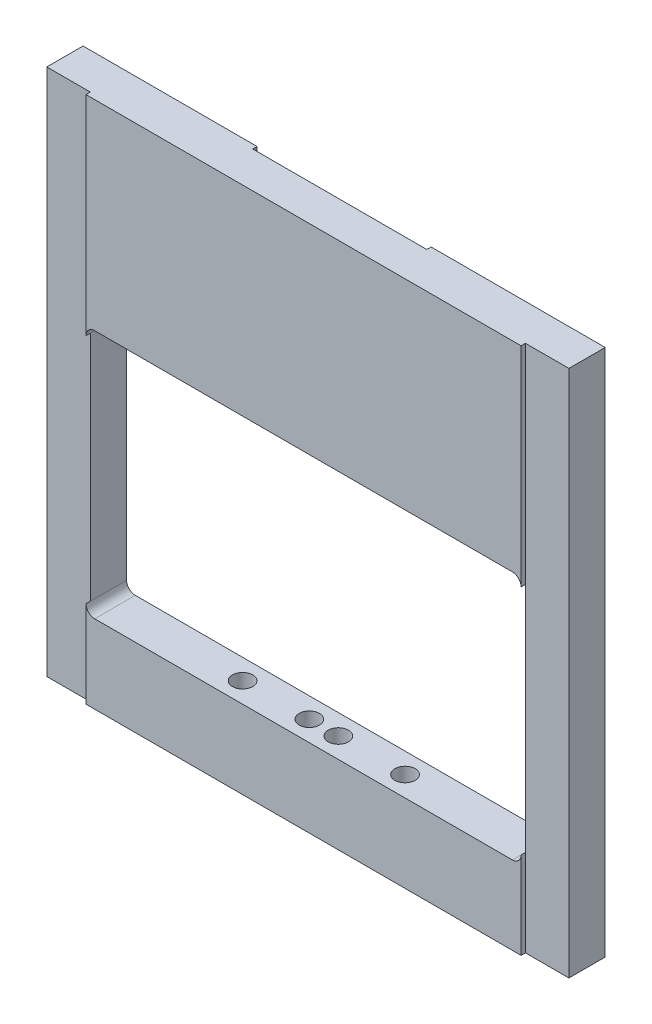
SolidWorks part; units mm, degrees
ref_plane "前视基准面" through (0, 0, 0) normal (0, 0, 1) x (1, 0, 0)
ref_plane "上视基准面" through (0, 0, 0) normal (0, 1, 0) x (1, 0, 0)
ref_plane "右视基准面" through (0, 0, 0) normal (1, 0, 0) x (0, 0, -1)
sketch "草图1" plane through (0, 0, 0) normal (0, 0, 1) x (1, 0, 0)
  line L1 (-90, -91) -> (90, -91)
  line L2 (-90, -91) -> (-90, 91)
  line L3 (-90, 91) -> (90, 91)
  line L4 (90, -91) -> (90, 91)
  line L5 (-90, -91) -> (90, 91) construction
  line L6 (-90, 91) -> (90, -91) construction
  point P0 (0, 0)
  dimension "D1" = 180
  dimension "D2" = 182
extrude "凸台-拉伸1" add sketch "草图1" along normal mid plane 14
sketch "草图2" plane through (0, 0, -7) normal (0, 0, -1) x (-1, 0, 0)
  line L0 (-90, 91) -> (90, 91) construction
  line L1 (-30, 27) -> (30, 27)
  line L2 (-30, 27) -> (-30, 91)
  line L3 (-30, 91) -> (30, 91)
  line L4 (30, 27) -> (30, 91)
  line L5 (-30, 27) -> (30, 91) construction
  line L6 (-30, 91) -> (30, 27) construction
  line L7 (90, -91) -> (-90, -91) construction
  line L8 (-30, -91) -> (30, -91)
  line L9 (-30, -91) -> (-30, -69)
  line L10 (-30, -69) -> (30, -69)
  line L11 (30, -91) -> (30, -69)
  line L12 (-30, -91) -> (30, -69) construction
  line L13 (-30, -69) -> (30, -91) construction
  point P0 (0, 59)
  point P7 (0, -80)
  dimension "D1" = 64
  dimension "D2" = 60
  dimension "D3" = 22
extrude "切除-拉伸1" cut sketch "草图2" against normal blind 1.5
sketch "草图3" plane through (0, 0, -7) normal (0, 0, -1) x (-1, 0, 0)
  line L0 (30, 27) -> (32, 27)
  line L1 (32, 37) -> (30, 37)
  line L2 (30, 27) -> (30, 91) construction
  line L3 (30, 37) -> (30, 27)
  line L9 (0, 0) -> (0, 27) construction
  line L10 (-30, 27) -> (30, 27) construction
  line L14 (-30, 37) -> (-30, 27)
  line L15 (-32, 37) -> (-30, 37)
  line L16 (-30, 27) -> (-32, 27)
  line L20 (30, -69) -> (32, -69)
  line L21 (32, -79) -> (30, -79)
  line L22 (30, -91) -> (30, -69) construction
  line L23 (30, -79) -> (30, -69)
  line L24 (-30, -79) -> (-30, -69)
  line L25 (-32, -79) -> (-30, -79)
  line L26 (-30, -69) -> (-32, -69)
  arc A0 (32, 27) -> (32, 37) centre (32, 32) ccw
  arc A3 (-32, 27) -> (-32, 37) centre (-32, 32) cw
  arc A4 (32, -69) -> (32, -79) centre (32, -74) cw
  arc A5 (-32, -69) -> (-32, -79) centre (-32, -74) ccw
  dimension "D1" = 5
  dimension "D3" = 5
  dimension "D2" = 2
  dimension "D4" = 2
extrude "切除-拉伸2" cut sketch "草图3" against normal up to surface (1.5 mm away) up to face at (0, -80, -5.5)
sketch "草图4" plane through (0, 0, -7) normal (0, 0, -1) x (-1, 0, 0)
  line L0 (-32, 27) -> (32, 27) construction
  line L1 (-75, -64) -> (75, -64)
  line L2 (-75, -64) -> (-75, 22)
  line L3 (-75, 22) -> (75, 22)
  line L4 (75, -64) -> (75, 22)
  line L5 (-75, -64) -> (75, 22) construction
  line L6 (-75, 22) -> (75, -64) construction
  line L7 (32, -69) -> (-32, -69) construction
  point P0 (0, -21)
  dimension "D1" = 150
  dimension "D2" = 5
  dimension "D3" = 5
extrude "切除-拉伸3" cut sketch "草图4" against normal up to next
fillet "圆角1" radius 3 4 edges at (75, 22, 0) (75, -64, 0) (-75, -64, 0) (-75, 22, 0)
sketch "草图6" plane through (0, -91, 0) normal (0, -1, 0) x (1, 0, 0)
  line L0 (-90, 7) -> (-90, -7) construction
  line L1 (90, 7) -> (90, -7) construction
  circle A0 centre (-28, 0) radius 3.5
  circle A1 centre (28, 0) radius 3.5
  circle A2 centre (-5, 0) radius 3.5
  circle A3 centre (5, 0) radius 3.5
extrude "切除-拉伸4" cut sketch "草图6" against normal up to next
sketch "草图7" plane through (0, 0, 7) normal (0, 0, 1) x (1, 0, 0)
  line L0 (-90, -91) -> (90, -91) construction
  line L1 (-90, 91) -> (-75, 91)
  line L2 (-90, 91) -> (-90, -91)
  line L3 (-90, -91) -> (-75, -91)
  line L4 (-75, 91) -> (-75, -91)
  line L6 (90, 91) -> (75, 91)
  line L7 (90, 91) -> (90, -91)
  line L8 (90, -91) -> (75, -91)
  line L9 (75, 91) -> (75, -91)
  dimension "D1" = 15
extrude "切除-拉伸5" cut sketch "草图7" against normal blind 1.5
equation "\"D6@草图6\"=\"D5@草图6\""
equation "\"D4@草图6\"=\"D3@草图6\""
